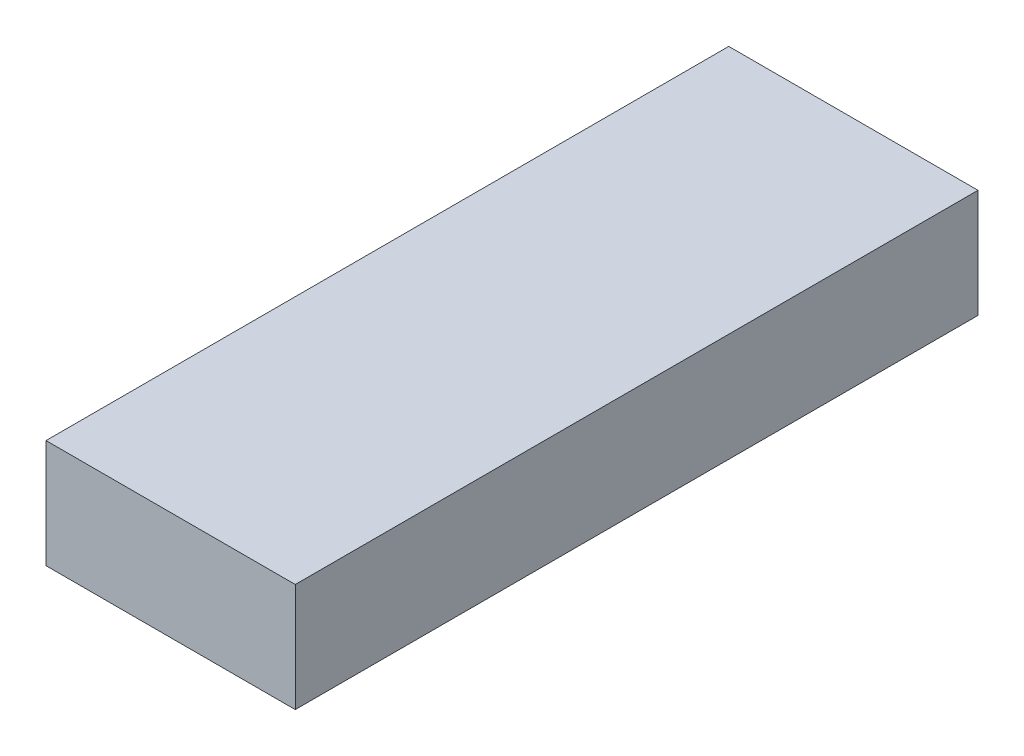
from build123d import *

# Parameters (mm, degrees)
SKETCH_1_W      = 23
SKETCH_1_H      = 63
EXTRUDE_1_DEPTH = 10


with BuildPart() as part:
    # 草图1 → 凸台-拉伸1 (new body)
    with BuildSketch(Plane(origin=(0, 0, 0), x_dir=(1, 0, 0), z_dir=(0, 1, 0))):
        with Locations((11.5, 31.5)):
            Rectangle(SKETCH_1_W, SKETCH_1_H)
    extrude(amount=EXTRUDE_1_DEPTH)


solid = part.part
